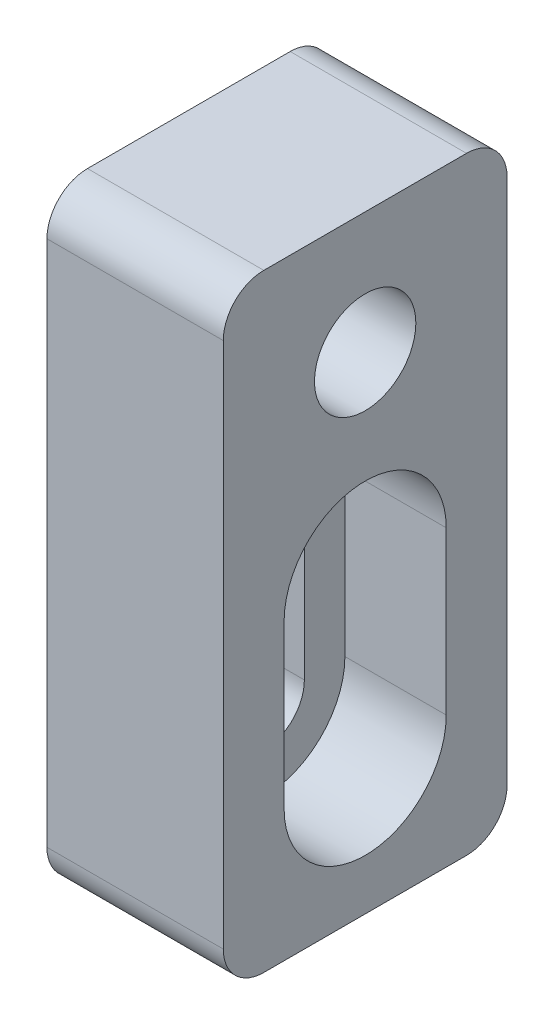
SolidWorks part; units mm, degrees
ref_plane "前视基准面" through (0, 0, 0) normal (0, 0, 1) x (1, 0, 0)
ref_plane "上视基准面" through (0, 0, 0) normal (0, 1, 0) x (1, 0, 0)
ref_plane "右视基准面" through (0, 0, 0) normal (1, 0, 0) x (0, 0, -1)
sketch "草图1" plane through (0, 0, 0) normal (0, 0, 1) x (1, 0, 0)
  line L1 (-4.35, 15) -> (4.35, 15)
  line L2 (-4.35, 15) -> (-4.35, -15)
  line L3 (-4.35, -15) -> (4.35, -15)
  line L4 (4.35, 15) -> (4.35, -15)
  line L5 (-4.35, 15) -> (4.35, -15) construction
  line L6 (-4.35, -15) -> (4.35, 15) construction
  point P0 (0, 0)
  dimension "D1" = 30
  dimension "D2" = 8.7
extrude "凸台-拉伸1" add sketch "草图1" along normal blind 14
hole_wizard "M6 螺纹孔1" positions "草图3" profile "草图2" tap size "M6" standard "Iso" end condition through all
sketch "草图3" plane through (4.35, 0, 0) normal (1, 0, 0) x (0, 0, -1)
  line L0 (-14, 15) -> (0, 15) construction
  point P0 (-7, 9)
  dimension "D1" = 6
sketch "草图2" plane through (4.35, 9, 7) normal (0, 1, 0) x (0, 0, -1)
  line L0 (0, 0) -> (0, 8.7)
  line L1 (0, 8.7) -> (2.5, 8.7)
  line L2 (2.5, 8.7) -> (2.5, 0)
  line L5 (2.5, 0) -> (0, 0)
  line L11 (0, -6.35) -> (0, 107.95) construction
  dimension "通孔螺纹孔钻头直径" = 5
  dimension "通孔螺纹孔钻头深度" = 8.7
cosmetic thread "孔螺蚊线1" parameters "D2"=6
sketch "草图4" plane through (4.35, 0, 0) normal (1, 0, 0) x (0, 0, -1)
  line L0 (-7, -8.5) -> (-7, -0.5) construction
  line L1 (-9, -8.5) -> (-9, -0.5)
  line L2 (-5, -8.5) -> (-5, -0.5)
  line L3 (-14, -15) -> (0, -15) construction
  arc A0 (-9, -8.5) -> (-5, -8.5) centre (-7, -8.5) ccw
  arc A1 (-5, -0.5) -> (-9, -0.5) centre (-7, -0.5) ccw
  point P2 (-7, -4.5)
  point P9 (-7, -15)
  dimension "D1" = 2
  dimension "D2" = 6.5
  dimension "D3" = 8
extrude "切除-拉伸1" cut sketch "草图4" against normal through all
sketch "草图5" plane through (4.35, 0, 0) normal (1, 0, 0) x (0, 0, -1)
  line L0 (-7, -0.5) -> (-7, -8.5) construction
  line L1 (-3, -0.5) -> (-3, -8.5)
  line L2 (-11, -0.5) -> (-11, -8.5)
  arc A0 (-3, -0.5) -> (-11, -0.5) centre (-7, -0.5) ccw
  arc A1 (-11, -8.5) -> (-3, -8.5) centre (-7, -8.5) ccw
  point P4 (-7, -4.5)
  dimension "D1" = 4
extrude "切除-拉伸2" cut sketch "草图5" against normal blind 5
fillet "圆角1" radius 2 4 edges at (0, -15, 0) (0, -15, 14) (0, 15, 14) (0, 15, 0)
